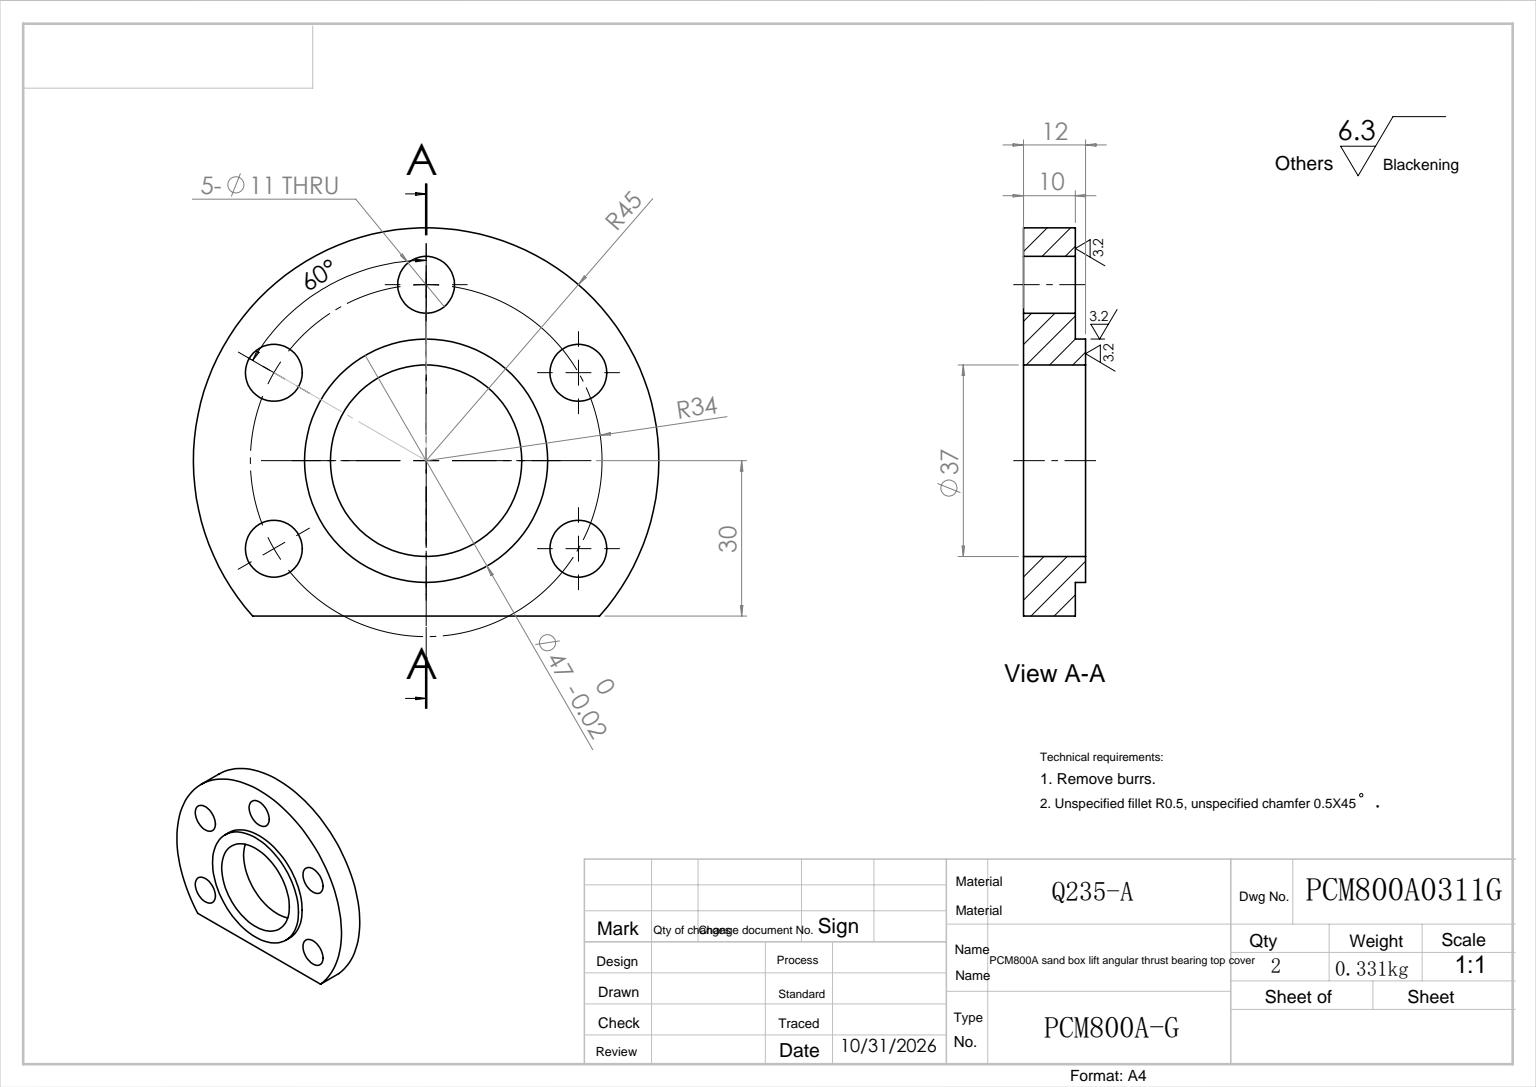
from build123d import *

# Parameters (mm, degrees)
SKETCH_1_R          = 45
SKETCH_1_R_2        = 18.5
EXTRUDE_1_DEPTH     = 10
SKETCH_2_R          = 23.5
SKETCH_2_R_2        = 18.5
EXTRUDE_2_DEPTH     = 2
SKETCH_3_R          = 5.5
CUT_EXTRUDE_1_DEPTH = 65.420493634
CUT_EXTRUDE_2_DEPTH = 65.420493634


with BuildPart() as part:
    # 草图1 → 拉伸1 (new body)
    with BuildSketch(Plane.XY):
        Circle(SKETCH_1_R)
        Circle(SKETCH_1_R_2, mode=Mode.SUBTRACT)
    extrude(amount=EXTRUDE_1_DEPTH)

    # 草图2 → 拉伸2 (add)
    with BuildSketch(Plane.XY.offset(10)):
        Circle(SKETCH_2_R)
        Circle(SKETCH_2_R_2, mode=Mode.SUBTRACT)
    extrude(amount=EXTRUDE_2_DEPTH)

    # 草图3 → 切除-拉伸1 (cut, through all)
    with BuildSketch(Plane.XY.offset(10)):
        with Locations((0, 34)):
            Circle(SKETCH_3_R)
        with Locations((-29.444863729, 17)):
            Circle(SKETCH_3_R)
        with Locations((-29.444863729, -17)):
            Circle(SKETCH_3_R)
        with Locations((29.444863729, 17)):
            Circle(SKETCH_3_R)
        with Locations((29.444863729, -17)):
            Circle(SKETCH_3_R)
    extrude(amount=-CUT_EXTRUDE_1_DEPTH, mode=Mode.SUBTRACT)

    # 草图4 → 切除-拉伸2 (cut, through all)
    with BuildSketch(Plane.XY.offset(10)):
        with BuildLine():
            Line((-35.388711425, -30), (35.388711425, -30))
            ThreePointArc((35.388711425, -30), (0, -46.393543692), (-35.388711425, -30))
        make_face()
    extrude(amount=-CUT_EXTRUDE_2_DEPTH, mode=Mode.SUBTRACT)


solid = part.part
